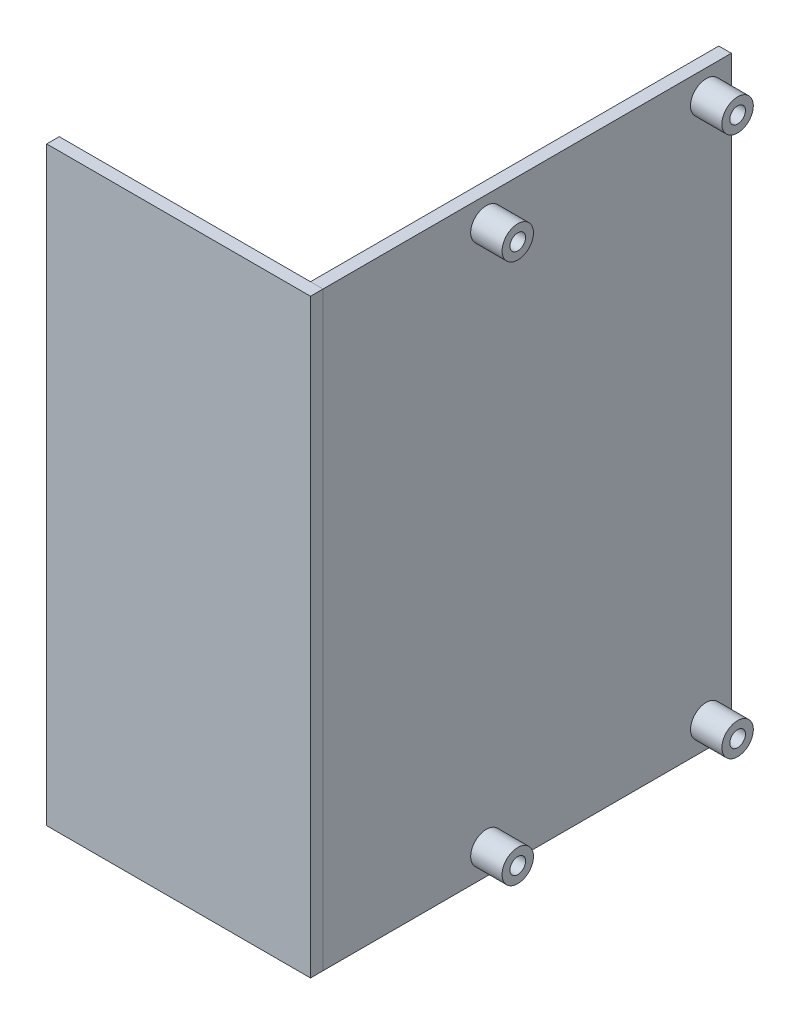
SolidWorks part; units mm, degrees
material "标准件"
ref_plane "前视基准面" through (0, 0, 0) normal (0, 0, 1) x (1, 0, 0)
ref_plane "上视基准面" through (0, 0, 0) normal (0, 1, 0) x (1, 0, 0)
ref_plane "右视基准面" through (0, 0, 0) normal (1, 0, 0) x (0, 0, -1)
sketch "草图1" plane through (0, 0, 0) normal (0, 0, 1) x (1, 0, 0)
  line L1 (-21, -47) -> (21, -47)
  line L2 (-21, -47) -> (-21, 47)
  line L3 (-21, 47) -> (21, 47)
  line L4 (21, -47) -> (21, 47)
  line L5 (-21, -47) -> (21, 47) construction
  line L6 (-21, 47) -> (21, -47) construction
  point P0 (0, 0)
  dimension "D1" = 42
  dimension "D2" = 94
extrude "凸台-拉伸1" add sketch "草图1" along normal blind 2
sketch "草图2" plane through (0, 0, 0) normal (0, 0, -1) x (-1, 0, 0)
  line L0 (21, -47) -> (-21, -47) construction
  line L1 (-21, 47) -> (-19, 47)
  line L2 (-21, 47) -> (-21, -47)
  line L3 (-21, -47) -> (-19, -47)
  line L4 (-19, 47) -> (-19, -47)
  dimension "D1" = 2
extrude "凸台-拉伸2" add sketch "草图2" along normal blind 65 separate body
sketch "草图3" plane through (21, 0, 0) normal (1, 0, 0) x (0, 0, -1)
  line L0 (0, 0) -> (68.5792, 0) construction
  line L1 (0, 47) -> (0, -47) construction
  line L2 (65, 47) -> (65, -47) construction
  circle A0 centre (26, 43) radius 2.5
  circle A1 centre (61, 43) radius 2.5
  circle A2 centre (61, -43) radius 2.5
  circle A3 centre (26, -43) radius 2.5
  dimension "D1" = 35
  dimension "D2" = 5
  dimension "D3" = 86
  dimension "D4" = 4
extrude "凸台-拉伸3" add sketch "草图3" along normal blind 5 separate body
hole_wizard "M3 螺纹孔1" positions "草图4" profile "草图5" tap size "M3" standard "ISO" end condition up to next
sketch "草图4" plane through (26, 0, 0) normal (1, 0, 0) x (0, 0, -1)
  point P0 (26, 43)
  point P3 (61, 43)
  point P6 (26, -43)
  point P9 (61, -43)
sketch "草图5" plane through (26, 43, -26) normal (0, 1, 0) x (0, 0, -1)
  line L0 (0, 0) -> (0, 5.001)
  line L1 (0, 5.001) -> (1.25, 5.001)
  line L2 (1.25, 5.001) -> (1.25, 0)
  line L5 (1.25, 0) -> (0, 0)
  line L11 (0, -6.35) -> (0, 107.95) construction
  dimension "通孔螺纹孔钻头直径" = 2.5
  dimension "通孔螺纹孔钻头深度" = 5.001
cosmetic thread "孔螺蚊线1" parameters "D2"=3
cosmetic thread "孔螺蚊线2" parameters "D2"=3
cosmetic thread "孔螺蚊线3" parameters "D2"=3
cosmetic thread "孔螺蚊线4" parameters "D2"=3
sketch "草图6" plane through (0, 0, 7) normal (0, 0, 1) x (1, 0, 0)
  line L0 (-30, 0) -> (30, 0) construction
  line L1 (-30, 60) -> (-30, -60) construction
  line L2 (30, -60) -> (30, 60) construction
  line L4 (-21, -47) -> (-1, -47)
  line L5 (-21, -47) -> (-21, 47)
  line L6 (-21, 47) -> (-1, 47)
  line L7 (-1, -47) -> (-1, 47)
  line L8 (-21, -47) -> (-1, 47) construction
  line L9 (-21, 47) -> (-1, -47) construction
  point P6 (-11, 0)
  point P11 (3.3254, 38.9905)
  point P12 (-21, 47)
  dimension "D1" = 20
extrude "切除-拉伸1" [suppressed] cut sketch "草图6" against normal up to next
